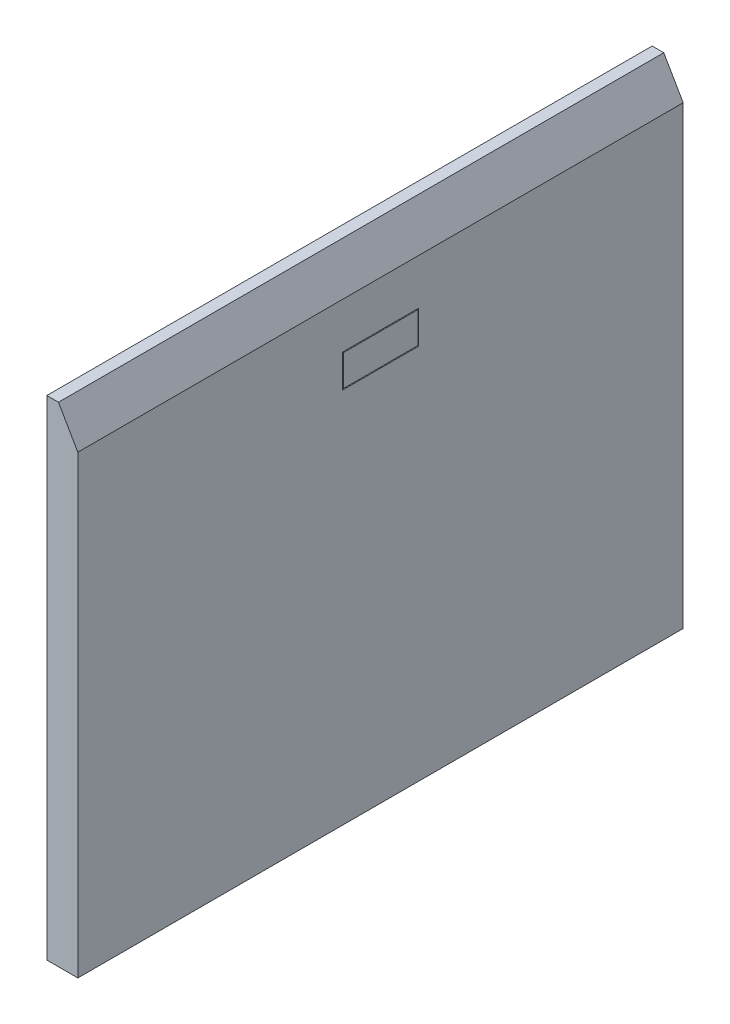
SolidWorks part; units mm, degrees
material "普通碳钢"
ref_plane "Front Plane" through (0, 0, 0) normal (0, 0, 1) x (1, 0, 0)
ref_plane "Top Plane" through (0, 0, 0) normal (0, 1, 0) x (1, 0, 0)
ref_plane "Right Plane" through (0, 0, 0) normal (1, 0, 0) x (0, 0, -1)
other "Configuration Table"
sketch "Sketch1" plane through (0, 0, 0) normal (0, 0, 1) x (1, 0, 0)
  line L0 (0, 0) -> (0, -630)
  line L1 (0, -630) -> (40, -630)
  line L2 (40, -630) -> (40, -43.3013)
  line L3 (0, 0) -> (15, 0)
  line L4 (15, 0) -> (40, -43.3013)
  dimension "D1" = 120
  dimension "D2" = 15
  dimension "D3" = 40
  dimension "D4" = 630
extrude "Boss-Extrude1" add sketch "Sketch1" along normal blind 780
sketch "Sketch2" plane through (40, 0, 0) normal (1, 0, 0) x (0, 0, -1)
  line L0 (-780, -43.3013) -> (0, -43.3013) construction
  line L1 (-438, -103.3013) -> (-342, -103.3013)
  line L2 (-438, -103.3013) -> (-438, -143.3013)
  line L3 (-438, -143.3013) -> (-342, -143.3013)
  line L4 (-342, -103.3013) -> (-342, -143.3013)
  line L5 (-390, -43.3013) -> (-390, -184.0153) construction
  point P8 (-390, -103.3013)
  dimension "D1" = 96
  dimension "D2" = 40
  dimension "D3" = 60
extrude "Cut-Extrude-Thin1" cut sketch "Sketch2" against normal blind 2 thin thin type one direction wall 1.2
